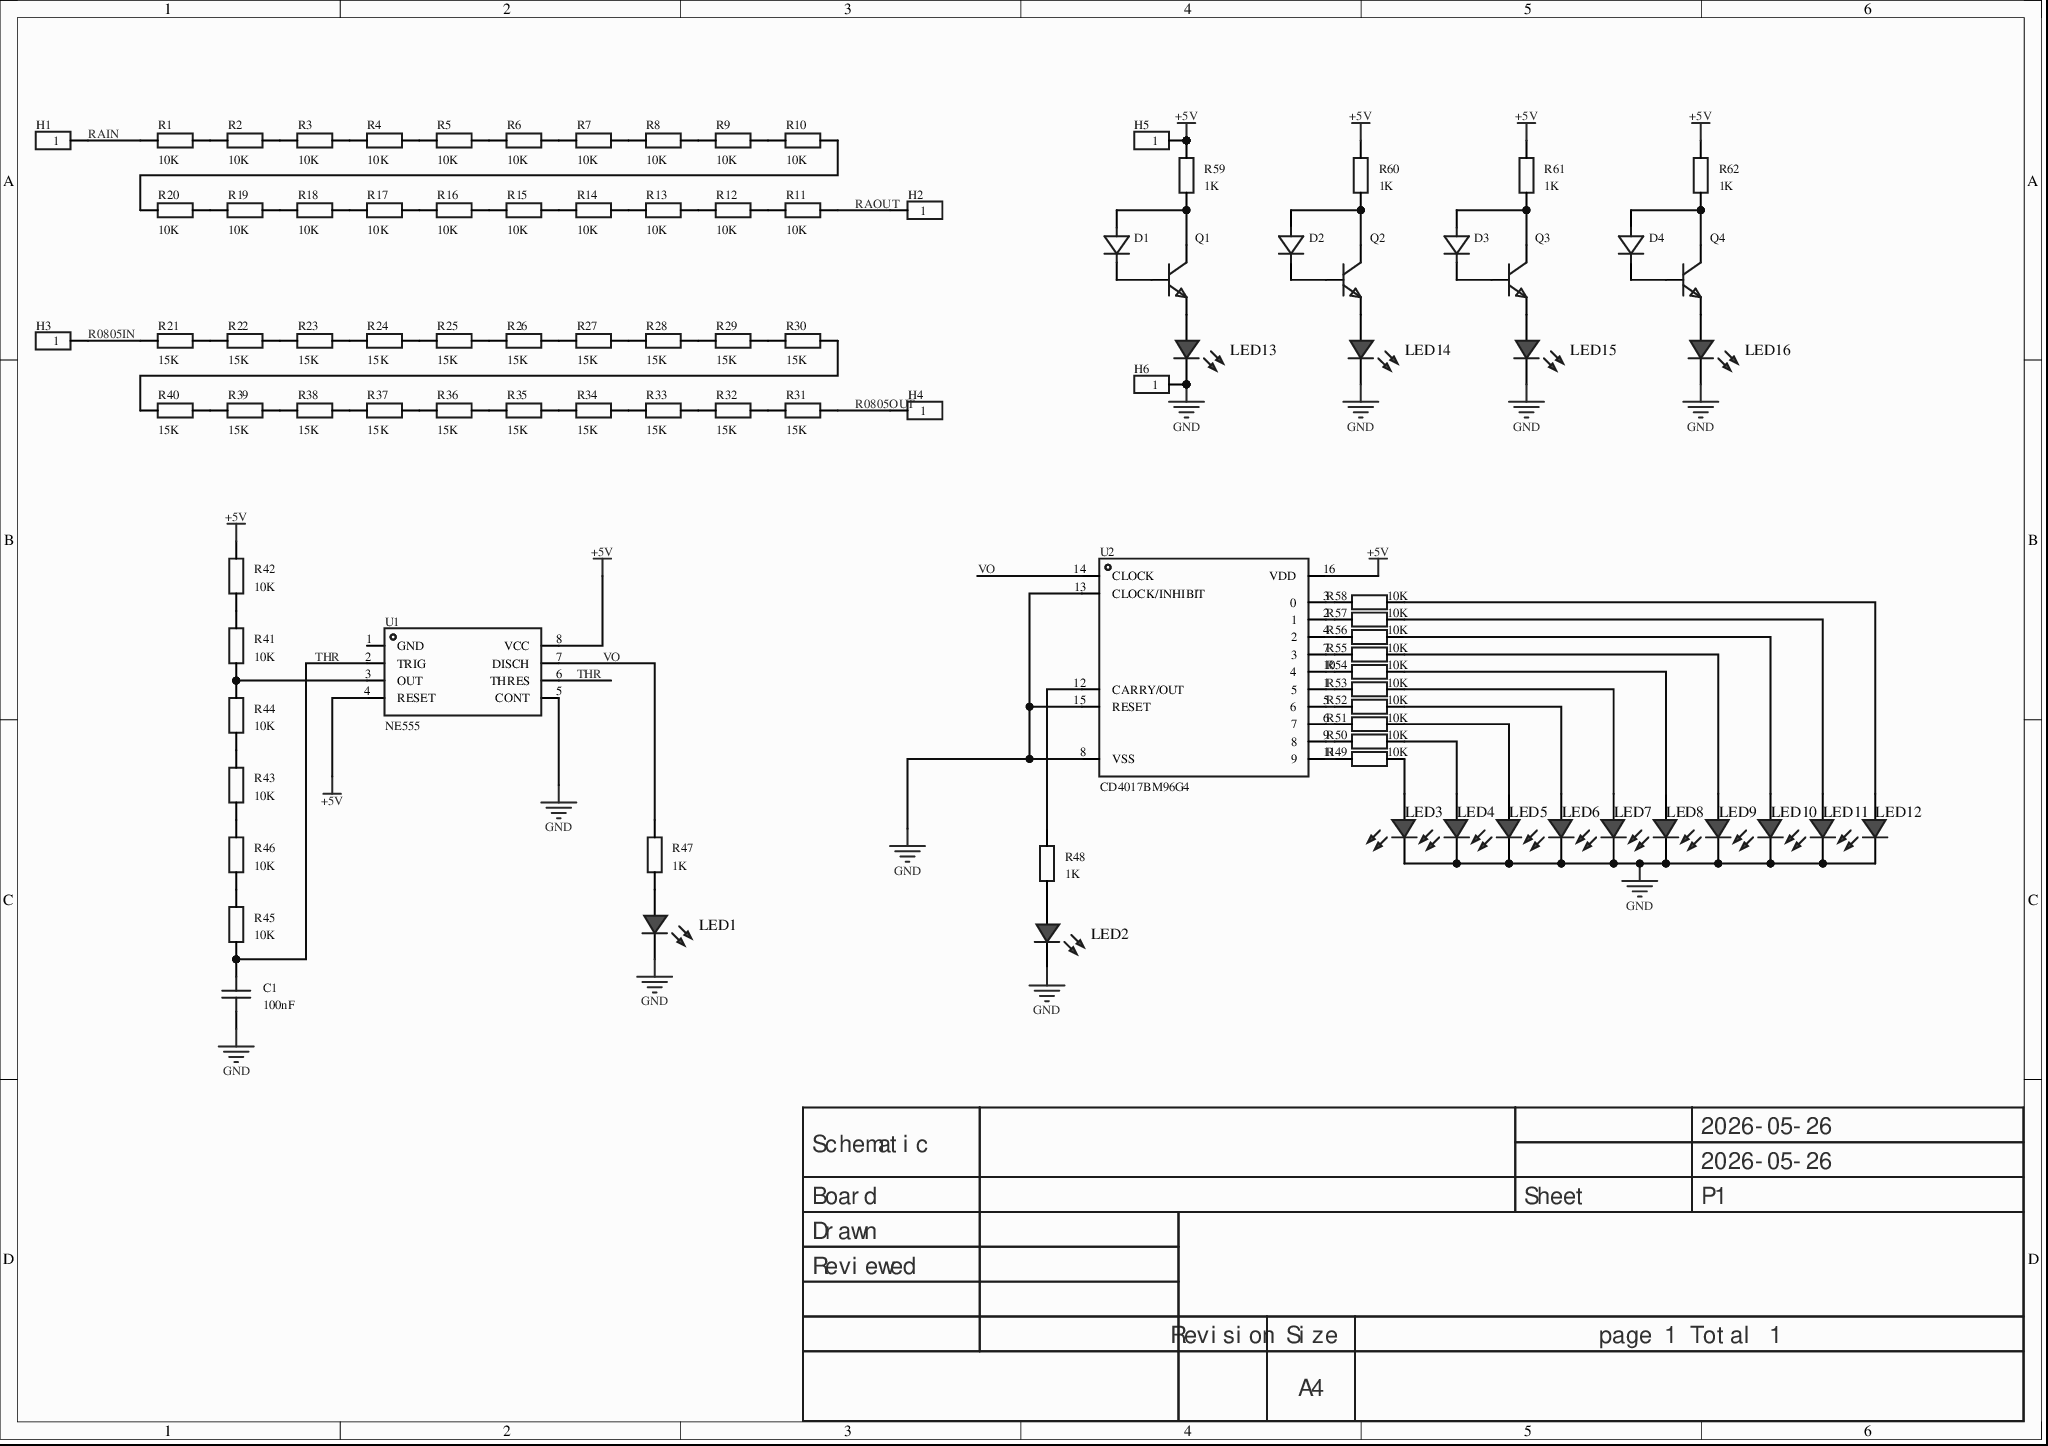
[diagram p0: MISC75384-3.schdoc]
# Altium project MISC75384-2.PrjPcb
1 sheet, 95 parts. Net scope: global (net labels, ports and power ports of the same name join across sheets).
Board file: MISC75384.pcbdoc

## Sheet MISC75384-3.schdoc
size 297 x 209 mm; Version: V1.0; @Project Name: MISC75384; @Update Date: 2026-05-26; @Create Date: 2026-05-26; @Board Name: MISC75384; @Create Time: 20:20:41; @Page Count: 1; @Page No: 1; @Schematic Name: MISC75384; @Update Time: 20:20:41; Size: A4

### Parts
C1  100nF  [C0805]
D1  (no value)  [SMA_1N4007]
D2  (no value)  [SMA_1N4007]
D3  (no value)  [SMA_1N4007]
D4  (no value)  [SMA_1N4007]
H1  (no value)  [HDR-TH_1P-V-M_XKB_X4611WV-01I-C28D40]
H2  (no value)  [HDR-TH_1P-V-M_XKB_X4611WV-01I-C28D40]
H3  (no value)  [HDR-TH_1P-V-M_XKB_X4611WV-01I-C28D40]
H4  (no value)  [HDR-TH_1P-V-M_XKB_X4611WV-01I-C28D40]
H5  (no value)  [HDR-TH_1P-V-M_XKB_X4611WV-01I-C28D40]
H6  (no value)  [HDR-TH_1P-V-M_XKB_X4611WV-01I-C28D40]
LED1  (no value)  [LED_0805]
LED2  (no value)  [LED_0805]
LED3  (no value)  [LED_0805]
LED4  (no value)  [LED_0805]
LED5  (no value)  [LED_0805]
LED6  (no value)  [LED_0805]
LED7  (no value)  [LED_0805]
LED8  (no value)  [LED_0805]
LED9  (no value)  [LED_0805]
LED10  (no value)  [LED_0805]
LED11  (no value)  [LED_0805]
LED12  (no value)  [LED_0805]
LED13  (no value)  [LED_0805]
LED14  (no value)  [LED_0805]
LED15  (no value)  [LED_0805]
LED16  (no value)  [LED_0805]
Q1  (no value)  [S8050_SOT-23]
Q2  (no value)  [S8050_SOT-23]
Q3  (no value)  [S8050_SOT-23]
Q4  (no value)  [S8050_SOT-23]
R1  10K  [R0805]
R2  10K  [R0805]
R3  10K  [R0805]
R4  10K  [R0805]
R5  10K  [R0805]
R6  10K  [R0805]
R7  10K  [R0805]
R8  10K  [R0805]
R9  10K  [R0805]
R10  10K  [R0805]
R11  10K  [R0805]
R12  10K  [R0805]
R13  10K  [R0805]
R14  10K  [R0805]
R15  10K  [R0805]
R16  10K  [R0805]
R17  10K  [R0805]
R18  10K  [R0805]
R19  10K  [R0805]
R20  10K  [R0805]
R21  15K  [R0805]
R22  15K  [R0805]
R23  15K  [R0805]
R24  15K  [R0805]
R25  15K  [R0805]
R26  15K  [R0805]
R27  15K  [R0805]
R28  15K  [R0805]
R29  15K  [R0805]
R30  15K  [R0805]
R31  15K  [R0805]
R32  15K  [R0805]
R33  15K  [R0805]
R34  15K  [R0805]
R35  15K  [R0805]
R36  15K  [R0805]
R37  15K  [R0805]
R38  15K  [R0805]
R39  15K  [R0805]
R40  15K  [R0805]
R41  10K  [R0805]
R42  10K  [R0805]
R43  10K  [R0805]
R44  10K  [R0805]
R45  10K  [R0805]
R46  10K  [R0805]
R47  1K  [R0805]
R48  1K  [R0805]
R49  10K  [R0805]
R50  10K  [R0805]
R51  10K  [R0805]
R52  10K  [R0805]
R53  10K  [R0805]
R54  10K  [R0805]
R55  10K  [R0805]
R56  10K  [R0805]
R57  10K  [R0805]
R58  10K  [R0805]
R59  1K  [R0805]
R60  1K  [R0805]
R61  1K  [R0805]
R62  1K  [R0805]
U1  NE555  [SOP-8_L5.0-W4.0-P1.27-LS6.0-BL]
U2  CD4017BM96G4  [SOIC-16_L9.9-W3.9-P1.27-LS6.0-BL]

### Nets
+5V: H5.1 R42.1 R59.2 R60.2 R61.2 R62.2 U1.4(RESET) U1.8(VCC) U2.16(VDD)
GND: C1.1 H6.1 LED1.1(C) LED2.1(C) LED3.1(C) LED4.1(C) LED5.1(C) LED6.1(C) LED7.1(C) LED8.1(C) LED9.1(C) LED10.1(C) LED11.1(C) LED12.1(C) LED13.1(C) LED14.1(C) LED15.1(C) LED16.1(C) U1.5(CONT) U2.8(VSS) U2.13(CLOCK/INHIBIT) U2.15(RESET)
R0805IN: H3.1 R21.1
R0805OUT: H4.1 R31.1
RAIN: H1.1 R1.1
RAOUT: H2.1 R11.1
THR: C1.2 R45.2 U1.2(TRIG) U1.6(THRES)
VO: R47.1 U1.7(DISCH) U2.14(CLOCK)
NetD1_1: D1.1(K) Q1.1
NetD1_2: D1.2(A) Q1.3 R59.1
NetD2_1: D2.1(K) Q2.1
NetD2_2: D2.2(A) Q2.3 R60.1
NetD3_1: D3.1(K) Q3.1
NetD3_2: D3.2(A) Q3.3 R61.1
NetD4_1: D4.1(K) Q4.1
NetD4_2: D4.2(A) Q4.3 R62.1
NetLED1_2: LED1.2(A) R47.2
NetLED2_2: LED2.2(A) R48.1
NetLED3_2: LED3.2(A) R49.2
NetLED4_2: LED4.2(A) R50.2
NetLED5_2: LED5.2(A) R51.2
NetLED6_2: LED6.2(A) R52.2
NetLED7_2: LED7.2(A) R53.2
NetLED8_2: LED8.2(A) R54.2
NetLED9_2: LED9.2(A) R55.2
NetLED10_2: LED10.2(A) R56.2
NetLED11_2: LED11.2(A) R57.2
NetLED12_2: LED12.2(A) R58.2
NetLED13_2: LED13.2(A) Q1.2
NetLED14_2: LED14.2(A) Q2.2
NetLED15_2: LED15.2(A) Q3.2
NetLED16_2: LED16.2(A) Q4.2
NetR1_2: R1.2 R2.1
NetR2_2: R2.2 R3.1
NetR3_2: R3.2 R4.1
NetR4_2: R4.2 R5.1
NetR5_2: R5.2 R6.1
NetR6_2: R6.2 R7.1
NetR7_2: R7.2 R8.1
NetR8_2: R8.2 R9.1
NetR9_2: R9.2 R10.1
NetR10_2: R10.2 R20.2
NetR11_2: R11.2 R12.1
NetR12_2: R12.2 R13.1
NetR13_2: R13.2 R14.1
NetR14_2: R14.2 R15.1
NetR15_2: R15.2 R16.1
NetR16_2: R16.2 R17.1
NetR17_2: R17.2 R18.1
NetR18_2: R18.2 R19.1
NetR19_2: R19.2 R20.1
NetR21_2: R21.2 R22.1
NetR22_2: R22.2 R23.1
NetR23_2: R23.2 R24.1
NetR24_2: R24.2 R25.1
NetR25_2: R25.2 R26.1
NetR26_2: R26.2 R27.1
NetR27_2: R27.2 R28.1
NetR28_2: R28.2 R29.1
NetR29_2: R29.2 R30.1
NetR30_2: R30.2 R40.2
NetR31_2: R31.2 R32.1
NetR32_2: R32.2 R33.1
NetR33_2: R33.2 R34.1
NetR34_2: R34.2 R35.1
NetR35_2: R35.2 R36.1
NetR36_2: R36.2 R37.1
NetR37_2: R37.2 R38.1
NetR38_2: R38.2 R39.1
NetR39_2: R39.2 R40.1
NetR41_1: R41.1 R42.2
NetR41_2: R41.2 R44.1 U1.3(OUT)
NetR43_1: R43.1 R44.2
NetR43_2: R43.2 R46.1
NetR45_1: R45.1 R46.2
NetR48_2: R48.2 U2.12(CARRY/OUT)
NetR49_1: R49.1 U2.11(9)
NetR50_1: R50.1 U2.9(8)
NetR51_1: R51.1 U2.6(7)
NetR52_1: R52.1 U2.5(6)
NetR53_1: R53.1 U2.1(5)
NetR54_1: R54.1 U2.10(4)
NetR55_1: R55.1 U2.7(3)
NetR56_1: R56.1 U2.4(2)
NetR57_1: R57.1 U2.2(1)
NetR58_1: R58.1 U2.3(0)

Not connected (* = marked no-connect by the designer): U1 1(GND)

### Notes on the sheet
- 2026-05-26
- Schematic
- Board
- Sheet
- P1
- Drawn
- Reviewed
- Revision
- Size
- A4
- page 1 Total 1

### Library data of the parts
C1 = CAP_0805: Symbol: Capacitance; ConvertToPcb: yes; ModelId: 1ba041120af144c991958decab20d2410819f05c4eef4c71ace90d822a990e87; ModelName: C0805_L2.0-W1.3-H1.3; ModelTransform: 78.74,51.181,0,0,0,0,0,0.0005,0; Device: CAP_0805; AddInBom: yes; Supplier Footprint: 0805; FootprintName: C0805; Value: 100nF
D1-D4 = D_1N4007: AddInBom: yes; ModelId: 4f1e9ef2303f48b48aa8ce0cacf8d7b10819f05c4eef4c71ace90d822a990e87; ModelName: SMA_L4.4-W2.8-LS5.4-RD; ModelTransform: 204.7,102.4,82.7,0,0,0,0,0,0; Symbol: D_1N4007; Device: D_1N4007; ConvertToPcb: yes; FootprintName: SMA_1N4007; Supplier Footprint: SMA
H1-H6 = HDR-M_2.54_1x1P: Symbol: HDR_1x1; ConvertToPcb: yes; ModelId: 95857080d3cc4057a19a22ccce05e1710819f05c4eef4c71ace90d822a990e87; ModelTransform: 78.74,79.1337,0,0,0,0,0,0,-110.236; Device: HDR-M_2.54_1x1P; AddInBom: yes; SupplierPart: C81276; Supplier Footprint: 插件; FootprintName: HDR-TH_1P-V-M_XKB_X4611WV-01I-C28D40; JLCPCB Part Class: Extended Part; ModelName: HDR-TH_1P-V-M_XKB_X4611WV-01I-C28D40
LED1-LED16 = LED_0805-R: Symbol: LED_R; Convert to PCB: yes; 3D Model: 33fb9fca58e84f37a403ebeef4c28b770819f05c4eef4c71ace90d822a990e87; 3D Model Transform: 78.7,49.1,39.3,0,0,0,0,0,0; ModelName: LED-0805_R; Device: LED_0805-R; Add into BOM: yes; Supplier Footprint: 0805; FootprintName: LED_0805
Q1-Q4 = S8050_SOT_NPN: Symbol: NPN; ConvertToPcb: yes; ModelId: c62791f0466c4ae2a892c056b845b0ca0819f05c4eef4c71ace90d822a990e87; ModelName: SOT-23-3P_L2.9-W1.3-H1.0-LS2.4-P0.95; ModelTransform: 98.6,114.12,41.29,180,0,0,0,0,-3; Device: S8050_SOT_NPN; AddInBom: yes; Supplier Footprint: SOT-23; FootprintName: S8050_SOT-23
R1-R62 = Res_0805: Symbol: Resistor; ConvertToPcb: yes; ModelId: 37a81e68749a4138bd2dfa6897b24b850819f05c4eef4c71ace90d822a990e87; ModelName: R0805_L2.0-W1.3-H0.6; ModelTransform: 78.74,51.181,0,0,0,0,0,-0.0005,0; Device: Res_0805; AddInBom: yes; Supplier Footprint: 0805; FootprintName: R0805
  R1-R20 R41-R46 R49-R58: Value: 10K
  R21-R40: Value: 15K
  R47 R48 R59-R62: Value: 1K
U1 = NE555: AddInBom: yes; ModelId: a3315c1c78f949e6bb82c6eaca1c53c70819f05c4eef4c71ace90d822a990e87; ModelName: SOP-8_L5.0-W4.0-H1.8-LS6.2-P1.27; ModelTransform: 244.094,196.85,0,90,0,0,0,0,0; Symbol: NE555; Device: NE555; LCSC Part Name: NE555; SupplierPart: C504549; ManufacturerPart: NE555; Supplier Footprint: SOP-8-4.0mm; JLCPCB Part Class: Extended Part; Supplier: LCSC; ConvertToPcb: yes; FootprintName: SOP-8_L5.0-W4.0-P1.27-LS6.0-BL
U2 = CD4017BM96G4: Input type: standard CMOS; operating voltage: 3V~18V; number of elements: 1; sink current (IOL): 640uA; source current (IOH): 510uA;; Manufacturer: TI(德州仪器); AddInBom: yes; ModelId: c21ec766ec2643efb3352f8441994f4e0819f05c4eef4c71ace90d822a990e87; ModelName: SOIC-16_L9.9-W3.9-H1.8-LS6.0-P1.27; ModelTransform: 389.763,236.454,0,0,0,0,0,0,0; output type: Push-pull; Number of Elements: 1; Channel Type: Unidirectional; Logic Family: CD4000B; Quiescent Current: 5uA; Symbol: CD4017BM96G4; Device: CD4017BM96G4; LCSC Part Name: CMOS逻辑集成电路; SupplierPart: C22329334; ManufacturerPart: CD4017BM96G4; Supplier Footprint: -; JLCPCB Part Class: Extended Part; Datasheet: https://example.com/datasheet/CD4017BM96G4/23761364.html; Supplier: LCSC; ConvertToPcb: yes; FootprintName: SOIC-16_L9.9-W3.9-P1.27-LS6.0-BL; Input type: Standard CMOS; Voltage - Supply: 3V~18V; Current - Output Low(IOL): 640uA; Current - Output High(IOH): 510uA; Operating Temperature: -55℃~+125℃